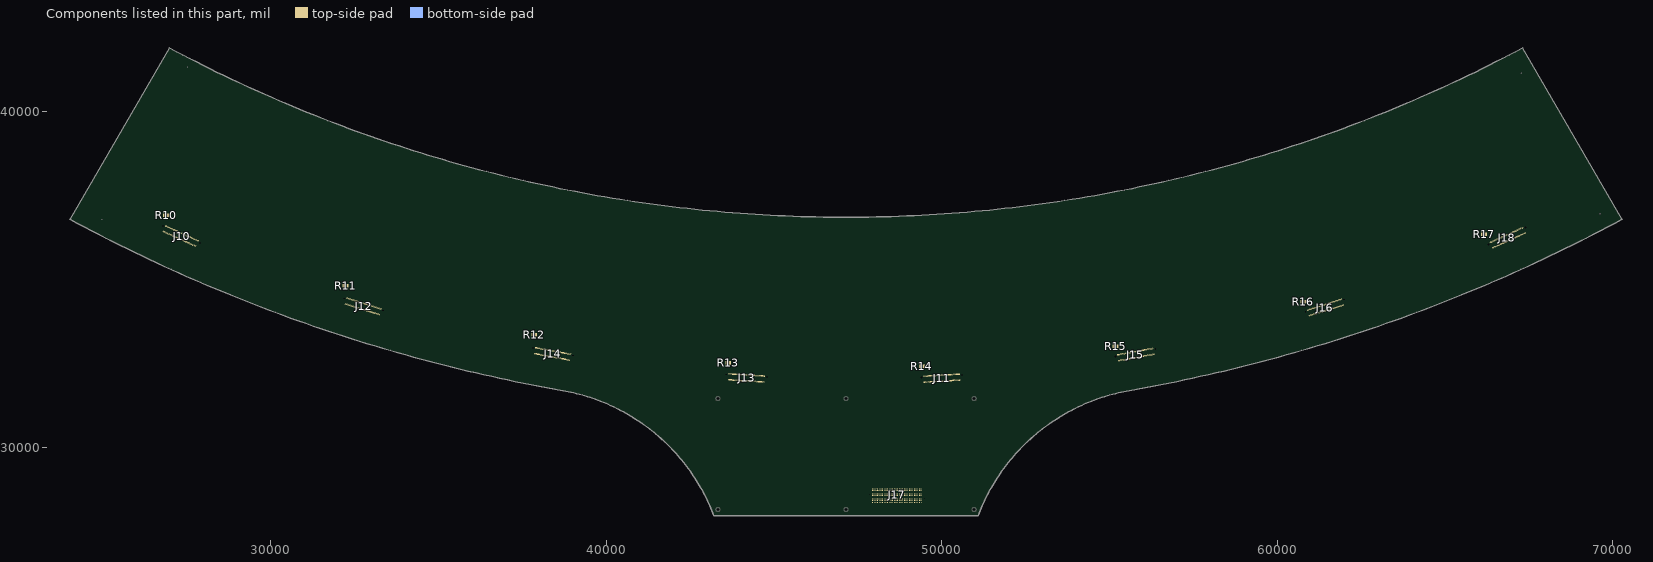
[diagram p0: the components of this part, seen from the top]
# Altium PCB MISC86329.PcbDoc (part 11 of 11)
Units mil, origin at the board's own origin, x right, y up, seen from the top; angles counter-clockwise.
Board outline 46247.15 x 13937.21 mil, 6 copper layers (Top Layer, GND2, SIG3, SIG4, POWER5, Bottom Layer); 17 components, 210 nets, 908 pads, 1109 vias.

## Polygon pours and split planes (outlines as drawn) (continued)
DGND on Bottom Layer "Top Layer-No Net" (solid, remove dead copper): 22045.95,43447.05 21968.95,43370.05 21968.95,25908.05 73506.95,25908.05 73814.95,26216.05 74045.95,26447.05 74045.95,43523.05 22121.95,43523.05 21968.95,43370.05
DGND on GND2 (split plane): 582 vertices, not listed, extent 24053.2,27990.2 70244.51,41880.36
5V_OUT on POWER5 (split plane): 582 vertices, not listed, extent 24053.2,27990.2 70244.51,41880.36

## Keep-outs
Keep-Out Layer:
  circle w3.94: c67272.94,41153 r59.06
  circle w3.94: c69620.94,36968 r59.06
  circle w3.94: c24972.94,36798 r59.06
  circle w3.94: c27525.94,41336 r59.06
  lines w5: 24025.43,36800.52 ccw(c47149,79657.81) 38712.02,31696.74 ; 24025.73,36800.35 26991.51,41907.14 ; 26991.25,41907.28 ccw(c47149,79657.81) 67306.76,41907.28 ; 38711.64,31696.8 cw(c37688.49,25880.6) 43212,27970.07 ; 43211.99,27970.1 51086.01,27970.1 ; 51086,27970.07 cw(c56609.51,25880.6) 55586.37,31696.8 ; 55585.98,31696.74 ccw(c47149,79657.81) 70272.58,36800.52 ; 67306.49,41907.14 70272.27,36800.35

## Silkscreen, mask and mechanical layers (free items; w line width, h text height)
Mechanical 1:
  drawing of 221 lines, arcs and shapes, not listed